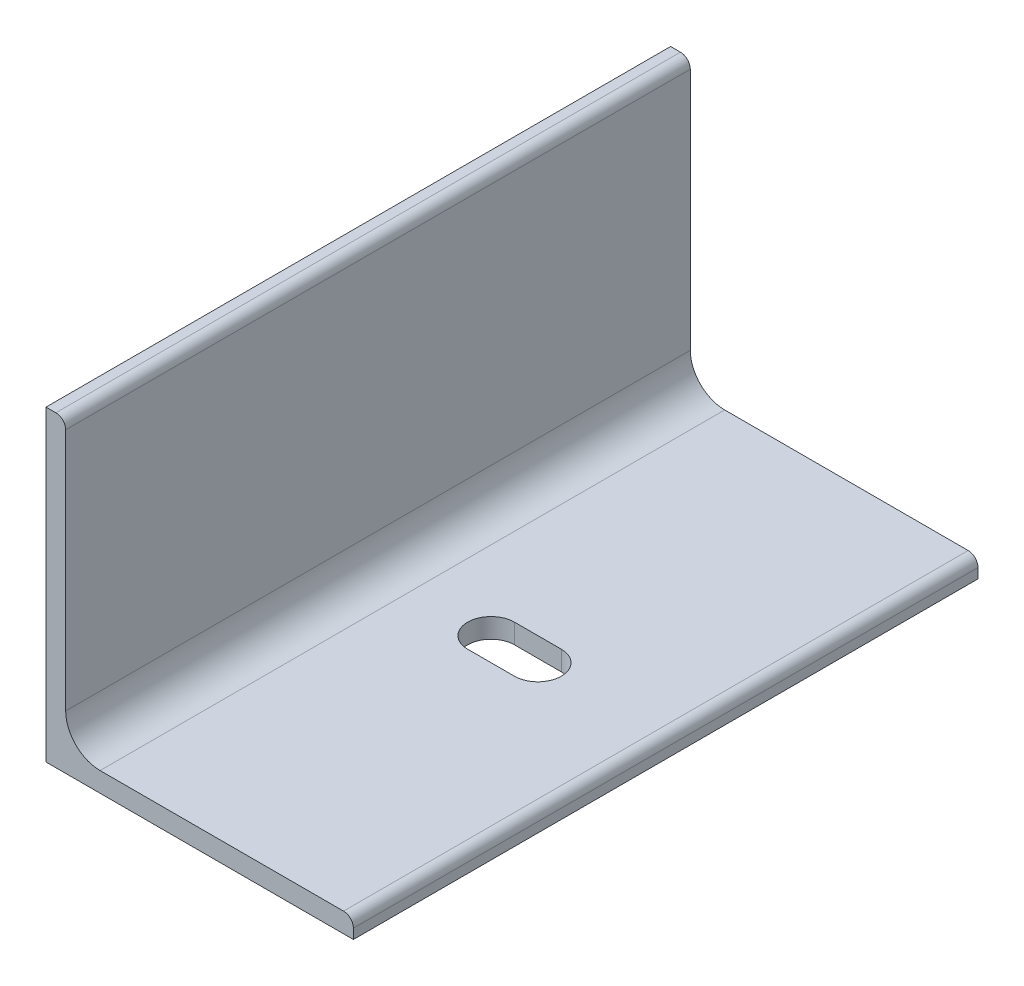
from build123d import *

# Parameters (mm, degrees)
BOSS_EXTRUDE1_DEPTH = 127
CUT_EXTRUDE1_DEPTH  = 304.8


with BuildPart() as part:
    # Sketch1 → Boss-Extrude1 (new, symmetric)
    with BuildSketch(Plane.XY):
        with BuildLine():
            Line((0, 125), (0, 0))
            Line((0, 0), (125, 0))
            Line((125, 0), (125, 4))
            ThreePointArc((125, 4), (123.828427125, 6.828427125), (121, 8))
            Line((121, 8), (22, 8))
            ThreePointArc((22, 8), (12.100505063, 12.100505063), (8, 22))
            Line((8, 22), (8, 121))
            ThreePointArc((8, 121), (6.828427125, 123.828427125), (4, 125))
            Line((4, 125), (0, 125))
        make_face()
    extrude(amount=BOSS_EXTRUDE1_DEPTH, both=True)

    # Sketch2 → Cut-Extrude1 (cut)
    with BuildSketch(Plane(origin=(0, 8, 0), x_dir=(1, 0, 0), z_dir=(0, 1, 0))):
        with BuildLine():
            Line((53.975, 9.525), (73.025, 9.525))
            ThreePointArc((73.025, 9.525), (82.55, 0), (73.025, -9.525))
            Line((73.025, -9.525), (53.975, -9.525))
            ThreePointArc((53.975, -9.525), (44.45, 0), (53.975, 9.525))
        make_face()
    extrude(amount=-CUT_EXTRUDE1_DEPTH, mode=Mode.SUBTRACT)


solid = part.part
